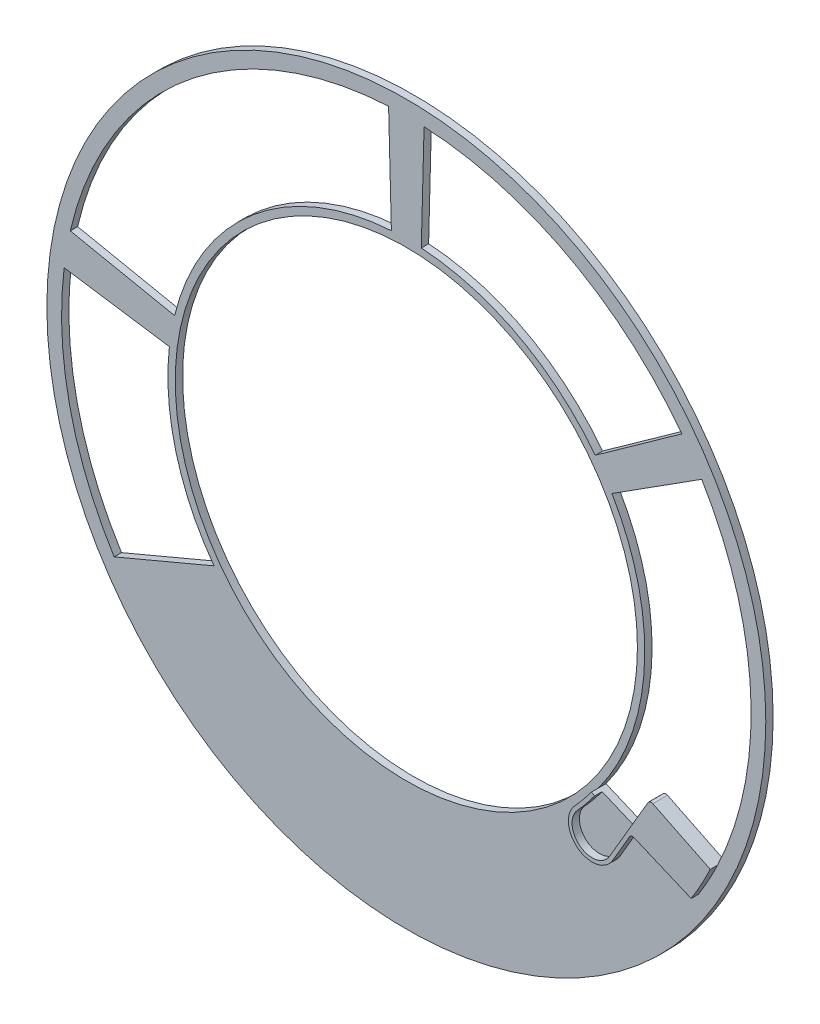
SolidWorks part; units mm, degrees
ref_plane "Front Plane" through (0, 0, 0) normal (0, 0, 1) x (1, 0, 0)
ref_plane "Top Plane" through (0, 0, 0) normal (0, 1, 0) x (1, 0, 0)
ref_plane "Right Plane" through (0, 0, 0) normal (1, 0, 0) x (0, 0, -1)
sketch "Sketch1" plane through (0, 0, 0) normal (0, 0, 1) x (1, 0, 0)
  circle A0 centre (0, 0) radius 98
  circle A1 centre (0, 0) radius 63
  dimension "D1" = 196
  dimension "D2" = 35
extrude "Boss-Extrude1" add sketch "Sketch1" along normal blind 2
sketch "Sketch2" plane through (0, 0, 2) normal (0, 0, 1) x (1, 0, 0)
  circle A0 centre (0, 0) radius 65
  circle A1 centre (0, 0) radius 63 construction
  circle A2 centre (0, 0) radius 94
  circle A3 centre (0, 0) radius 98 construction
  dimension "D1" = 2
  dimension "D2" = 4
extrude "Cut-Extrude2" cut sketch "Sketch2" against normal blind 5
sketch "Sketch3" plane through (0, 0, 2) normal (0, 0, 1) x (1, 0, 0)
  line L0 (0, 0) -> (0, 124.5571) construction
  line L1 (4.8362, 93.8755) -> (4.0768, 64.872)
  line L2 (-4.8362, 93.8755) -> (-4.0768, 64.872)
  line L15 (75.1219, 56.5039) -> (51.5017, 39.6558)
  line L16 (0, 0) -> (47.2242, 44.6641) construction
  line L19 (80.5307, 48.4851) -> (56.061, 32.8962)
  line L20 (88.8515, -30.6823) -> (61.6755, -20.5216) [skipped]
  line L21 (85.2282, -39.6505) -> (58.6211, -28.0814) [skipped]
  line L22 (24.2484, -90.8186) -> (17.4753, -62.6068) [skipped]
  line L23 (14.7873, -92.8296) -> (9.5, -64.302) [skipped]
  line L24 (-61.7325, -70.8879) -> (-42.1313, -49.497) [skipped]
  line L25 (-68.6903, -64.1689) -> (-47.9965, -43.8331) [skipped]
  line L26 (-93.2891, 11.5385) -> (-64.5944, 7.2501)
  line L27 (-91.6095, 21.0641) -> (-63.1786, 15.2797)
  line L28 (0, 0) -> (4.0768, 64.872) construction
  line L29 (0, 0) -> (56.061, 32.8962) construction
  circle A0 centre (0, 0) radius 65 construction
  arc A1 (4.0768, 64.872) -> (-4.0768, 64.872) centre (0, 0) ccw
  circle A2 centre (0, 0) radius 94 construction
  arc A3 (4.8362, 93.8755) -> (-4.8362, 93.8755) centre (0, 0) ccw
  arc A18 (80.5307, 48.4851) -> (75.1219, 56.5039) centre (0, 0) ccw
  arc A19 (56.061, 32.8962) -> (51.5017, 39.6558) centre (0, 0) ccw
  arc A20 (85.2282, -39.6505) -> (88.8515, -30.6823) centre (0, 0) ccw [skipped]
  arc A21 (58.6211, -28.0814) -> (61.6755, -20.5216) centre (0, 0) ccw [skipped]
  arc A22 (14.7873, -92.8296) -> (24.2484, -90.8186) centre (0, 0) ccw [skipped]
  arc A23 (9.5, -64.302) -> (17.4753, -62.6068) centre (0, 0) ccw [skipped]
  arc A24 (-68.6903, -64.1689) -> (-61.7325, -70.8879) centre (0, 0) ccw [skipped]
  arc A25 (-47.9965, -43.8331) -> (-42.1313, -49.497) centre (0, 0) ccw [skipped]
  arc A26 (-91.6095, 21.0641) -> (-93.2891, 11.5385) centre (0, 0) ccw
  arc A27 (-63.1786, 15.2797) -> (-64.5944, 7.2501) centre (0, 0) ccw
  point P32 (0, 0)
  dimension "D1" = 6
  dimension "D2" = 56
extrude "Boss-Extrude2" add sketch "Sketch3" against normal blind 2
sketch "Sketch8" plane through (0, 0, 2) normal (0, 0, 1) x (1, 0, 0)
  line L0 (-52.4241, -38.4281) -> (-79.65, -49.9187)
  line L1 (0, 0) -> (0, -143.5703) construction
  line L2 (52.4241, -38.4281) -> (79.65, -49.9187)
  arc A0 (-64.5944, 7.2501) -> (56.061, 32.8962) centre (0, 0) ccw construction
  arc A1 (-52.4241, -38.4281) -> (52.4241, -38.4281) centre (0, 0) ccw
  arc A2 (-93.2891, 11.5385) -> (80.5307, 48.4851) centre (0, 0) ccw construction
  arc A3 (-79.65, -49.9187) -> (79.65, -49.9187) centre (0, 0) ccw
extrude "Boss-Extrude7" add sketch "Sketch8" against normal blind 2
sketch "Sketch9" plane through (0, 0, 2) normal (0, 0, 1) x (1, 0, 0)
  line L1 (57.3968, -51.1014) -> (67.887, -33.166)
  line L2 (58.26, -51.6063) -> (68.2812, -34.4726)
  line L3 (69.5843, -34.0794) -> (84.4192, -41.3449)
  line L4 (69.19, -32.7728) -> (84.859, -40.4469)
  line L5 (79.65, -49.9187) -> (52.4241, -38.4281) construction
  line L6 (79.65, -49.9187) -> (63.2864, -43.0125)
  line L7 (53.3706, -38.8276) -> (52.4241, -38.4281)
  line L8 (58.26, -51.6063) -> (68.7502, -33.6709) construction
  line L9 (68.7502, -33.6709) -> (84.4192, -41.3449) construction
  line L10 (68.3559, -32.3643) -> (84.859, -40.4469) construction
  line L11 (57.3968, -51.1014) -> (68.3559, -32.3643) construction
  arc A0 (52.4241, -38.4281) -> (56.061, 32.8962) centre (0, 0) ccw construction
  arc A1 (47.8889, -43.9506) -> (52.4241, -38.4281) centre (0, 0) ccw
  arc A2 (47.8889, -43.9506) -> (58.26, -51.6063) centre (52.6646, -48.3336) ccw
  arc A4 (79.65, -49.9187) -> (80.5307, 48.4851) centre (0, 0) ccw construction
  arc A5 (48.6256, -44.6268) -> (53.3706, -38.8276) centre (0, 0) ccw
  arc A6 (48.6256, -44.6268) -> (57.3968, -51.1014) centre (52.6646, -48.3336) ccw
  arc A7 (48.6256, -44.6268) -> (53.2306, -39.0193) centre (0, 0) ccw construction
  arc A8 (84.4192, -41.3449) -> (84.8542, -40.4445) centre (0, 0) ccw
  arc A9 (68.2812, -34.4726) -> (69.5843, -34.0794) centre (69.1444, -34.9775) cw
  arc A10 (69.19, -32.7728) -> (67.887, -33.166) centre (68.7502, -33.6709) ccw
  arc A11 (79.65, -49.9187) -> (84.8542, -40.4445) centre (0, 0) ccw
  line M6 (79.65, -49.9187) -> (52.4241, -38.4281)
  arc M9 (80.5307, 48.4851) -> (79.65, -49.9187) centre (0, 0) cw
  dimension "D1" = 1
  dimension "D2" = 1
extrude "Boss-Extrude9" add sketch "Sketch9" along normal mid plane 4 contours A9 L2 L3 M6 M9 | L4 A10 L1 L2 A9 L3 M6 M9 | A6 A5 A1 A2 L2 L1 M6
fillet "Fillet1" radius 1 1 edges at (63.2864, -43.0125, 3)
